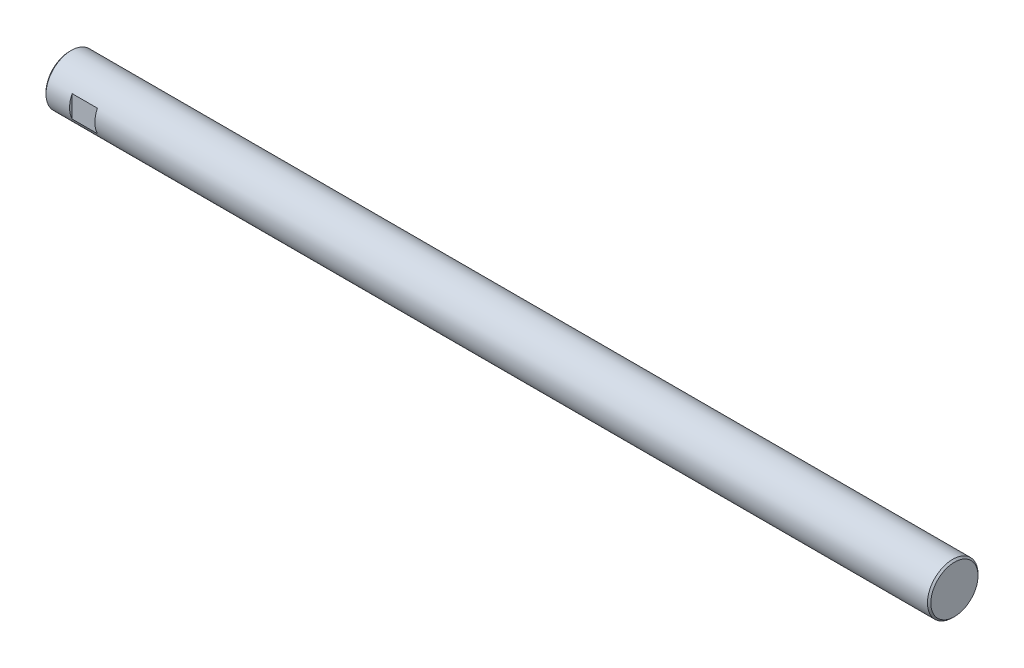
SolidWorks part; units mm, degrees
material "GCr15 (Cr)"
ref_plane "Front Plane" through (0, 0, 0) normal (0, 0, 1) x (1, 0, 0)
ref_plane "Top Plane" through (0, 0, 0) normal (0, 1, 0) x (1, 0, 0)
ref_plane "Right Plane" through (0, 0, 0) normal (1, 0, 0) x (0, 0, -1)
sketch "Sketch1" plane through (0, 0, 0) normal (0, 0, 1) x (1, 0, 0)
  line L0 (0, 0) -> (0, 14)
  line L1 (0, 14) -> (1, 15)
  line L2 (1, 15) -> (524, 15)
  line L3 (524, 15) -> (525, 14)
  line L4 (525, 14) -> (525, 0)
  line L5 (525, 0) -> (0, 0)
  line L6 (525, 0) -> (0, 0) construction
  dimension "D1" = 15
  dimension "D2" = 525
  dimension "D3" = 1
  dimension "D4" = 1
revolve "Revolve1" add sketch "Sketch1" angle 360 about L6
sketch "Sketch2" plane through (0, 0, 0) normal (0, 0, 1) x (1, 0, 0)
  line L0 (0, 0) -> (0, 4)
  line L1 (0, 4) -> (0.6765, 3.3235)
  line L2 (0.6765, 3.3235) -> (17.6, 3.3235)
  line L3 (17.6, 3.3235) -> (19.5188, 0)
  line L4 (19.5188, 0) -> (0, 0)
  line L5 (19.5188, 0) -> (0, 0) construction
revolve "Cut-Revolve1" cut sketch "Sketch2" angle 360 about L5
cosmetic thread "Cosmetic Thread1" parameters "D1"=16, "D2"=8
ref_plane "Plane1" through (15, 0, 0) normal (1, 0, 0) x (0, 0, -1)
sketch "Sketch3" plane through (15, 0, 0) normal (1, 0, 0) x (0, 0, -1)
  line L0 (-27, -60) -> (27, -60)
  line L1 (27, -60) -> (27, 60)
  line L2 (27, 60) -> (-27, 60)
  line L3 (-27, 60) -> (-27, -60)
  line L4 (-13.5, -30) -> (13.5, -30)
  line L5 (13.5, -30) -> (13.5, 30)
  line L6 (13.5, 30) -> (-13.5, 30)
  line L7 (-13.5, 30) -> (-13.5, -30)
extrude "Cut-Extrude1" cut sketch "Sketch3" along normal blind 15
ref_plane "Plane2" through (0, 15, 0) normal (0, 1, 0) x (1, 0, 0)
ref_plane "Plane3" through (0, 0, 15) normal (0, 0, 1) x (1, 0, 0)
ref_plane "Plane4" through (360, 0, 0) normal (1, 0, 0) x (0, 0, -1)
